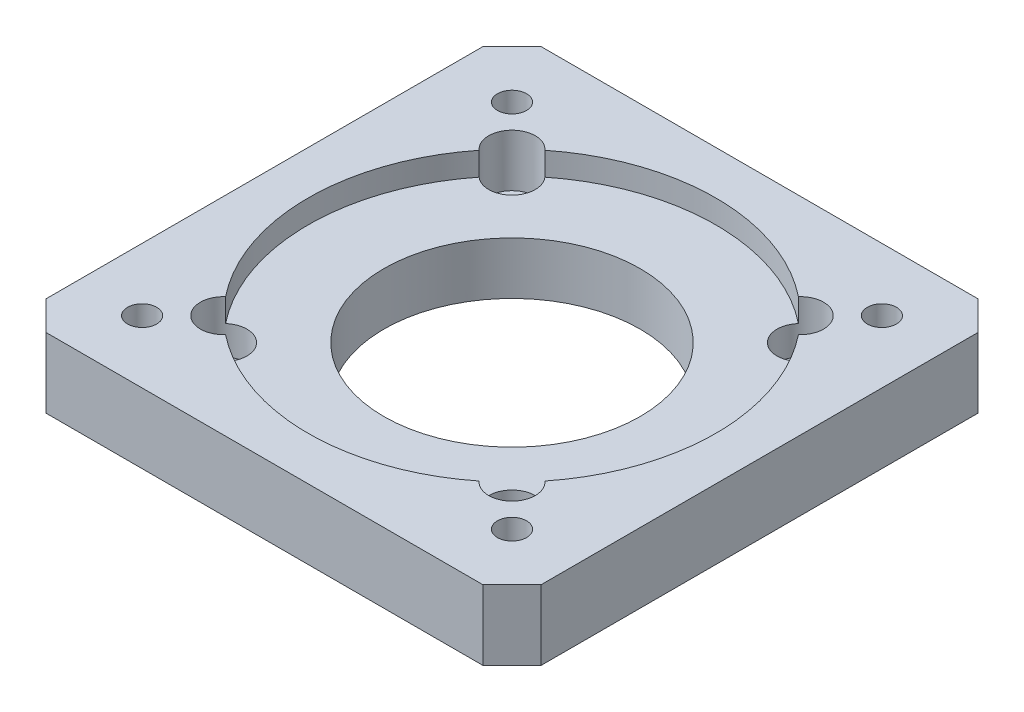
from build123d import *

# Parameters (mm, degrees)
SKETCH_1_W             = 85
SKETCH_1_H             = 85
EXTRUDE_1_DEPTH        = 6
SKETCH_2_R             = 25
EXTRUDE_2_DEPTH        = 1
SKETCH_3_R             = 22
CUT_EXTRUDE_1_DEPTH    = 62.493902137
SKETCH_4_R             = 35
CUT_EXTRUDE_2_DEPTH    = 4
HOLE_WIZARD_M6_1_D     = 5
CHAMFER_1_SIZE         = 5
PZ_000000C_D           = 4.5
PZ_000000C_CBORE_D     = 8
PZ_000000C_CBORE_DEPTH = 9


with BuildPart() as part:
    # 草图1 → 凸台-拉伸1 (new, symmetric)
    with BuildSketch(Plane(origin=(0, 0, 0), x_dir=(1, 0, 0), z_dir=(0, 1, 0))):
        Rectangle(SKETCH_1_W, SKETCH_1_H)
    extrude(amount=EXTRUDE_1_DEPTH, both=True)

    # 草图2 → 凸台-拉伸2 (add, symmetric)
    with BuildSketch(Plane.XZ.offset(6)):
        with Locations(Location((0, 0, 0), (0, 0, 270))):
            Circle(SKETCH_2_R)
    extrude(amount=EXTRUDE_2_DEPTH, both=True)

    # 草图3 → 切除-拉伸1 (cut, through all)
    with BuildSketch(Plane.XZ.offset(7)):
        with Locations(Location((0, 0, 0), (0, 0, 270))):
            Circle(SKETCH_3_R)
    extrude(amount=-CUT_EXTRUDE_1_DEPTH, mode=Mode.SUBTRACT)

    # 草图4 → 切除-拉伸2 (cut)
    with BuildSketch(Plane(origin=(0, 6, 0), x_dir=(1, 0, 0), z_dir=(0, 1, 0))):
        with Locations(Location((0, 0, 0), (0, 0, 270))):
            Circle(SKETCH_4_R)
    extrude(amount=-CUT_EXTRUDE_2_DEPTH, mode=Mode.SUBTRACT)

    # M6 螺纹孔1 (through all)
    with Locations(Plane(origin=(0, 6, 0), x_dir=(1, 0, 0), z_dir=(0, 1, 0))):
        with Locations((-31.75, 31.75), (0, 0), (31.75, -31.75), (31.75, 31.75), (-31.75, -31.75)):
            Hole(HOLE_WIZARD_M6_1_D / 2)

    # 倒角1
    chamfer_1_edges = [part.edges().sort_by_distance(p)[0] for p in [
        (42.5, 0, 42.5),
        (-42.5, 0, 42.5),
        (-42.5, 0, -42.5),
        (42.5, 0, -42.5),
    ]]
    chamfer(chamfer_1_edges, length=CHAMFER_1_SIZE)

    # PZ-000000C 铺砖车 (through all)
    with Locations(Plane(origin=(0, 6, 0), x_dir=(1, 0, 0), z_dir=(0, 1, 0))):
        with Locations((-24.748737342, 24.748737341), (24.748737342, 24.748737342), (24.748737342, -24.748737342), (-24.748737342, -24.748737342)):
            CounterBoreHole(PZ_000000C_D / 2, PZ_000000C_CBORE_D / 2, PZ_000000C_CBORE_DEPTH)


solid = part.part
